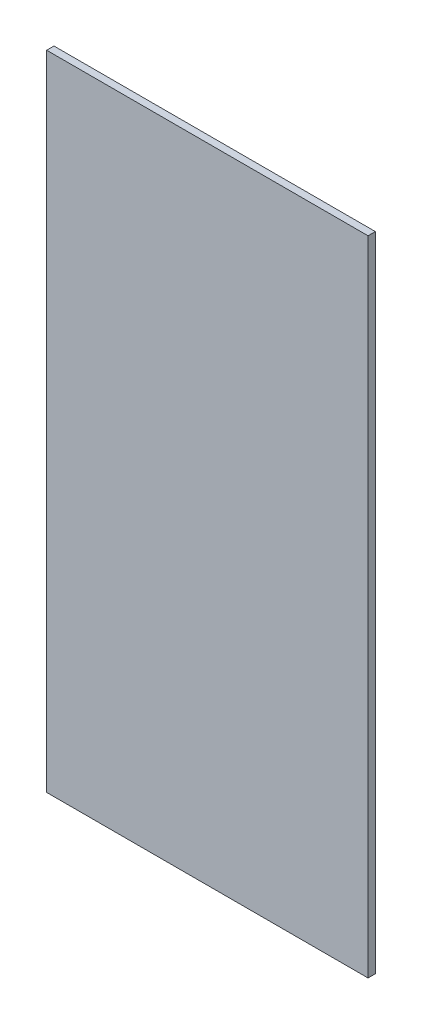
from build123d import *

# Parameters (mm, degrees)
SKETCH_1_W      = 44
SKETCH_1_H      = 88
EXTRUDE_1_DEPTH = 0.5


with BuildPart() as part:
    # 草图1 → 凸台-拉伸1 (new, symmetric)
    with BuildSketch(Plane.XY):
        Rectangle(SKETCH_1_W, SKETCH_1_H)
    extrude(amount=EXTRUDE_1_DEPTH, both=True)


solid = part.part
